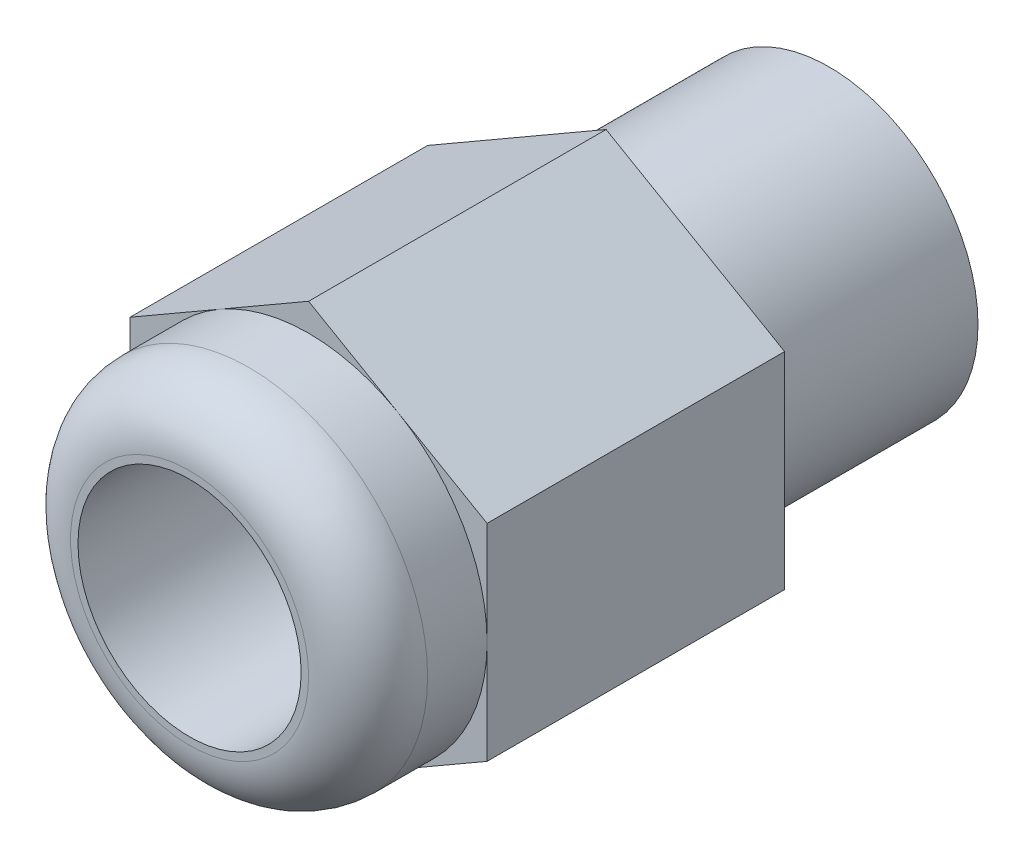
from build123d import *
from build123d.topology import SkipClean

# Parameters (mm, degrees)
SKETCH_1_R      = 7.5
EXTRUDE_1_DEPTH = 20
SKETCH_3_R      = 12
SKETCH_3_R_2    = 7.5
EXTRUDE_3_DEPTH = 8
FILLET_1_R      = 4
EXTRUDE_START   = 15
SKETCH_4_R      = 10
SKETCH_4_R_2    = 7.5
EXTRUDE_4_DEPTH = 15


with BuildPart() as part:
    # 草图1 → 凸台-拉伸1 (new body)
    with BuildSketch(Plane.XY):
        Polygon((0, 13.856406461), (-12, 6.92820323), (-12, -6.92820323), (0, -13.856406461), (12, -6.92820323), (12, 6.92820323), align=None)
        Circle(SKETCH_1_R, mode=Mode.SUBTRACT)
    extrude(amount=EXTRUDE_1_DEPTH)

    # 草图3 → 凸台-拉伸3 (add)
    with BuildSketch(Plane.XY.offset(20)):
        Circle(SKETCH_3_R)
        Circle(SKETCH_3_R_2, mode=Mode.SUBTRACT)
    extrude(amount=EXTRUDE_3_DEPTH)

    # 圆角1
    fillet_1_edges = [part.edges().sort_by_distance(p)[0] for p in [
        (-12, 0, 28),
    ]]
    fillet(fillet_1_edges, radius=FILLET_1_R)

    # 草图4 → 凸台-拉伸4 (add)
    with SkipClean():  # the faces are left unmerged after this step: merging them gives an invalid solid
        with BuildSketch(Plane(origin=(0, 0, 0), x_dir=(-1, 0, 0), z_dir=(0, 0, -1)).offset(EXTRUDE_START)):
            with Locations(Location((0, 0, 0), (0, 0, 180))):
                Circle(SKETCH_4_R)
            Circle(SKETCH_4_R_2, mode=Mode.SUBTRACT)
        extrude(amount=-EXTRUDE_4_DEPTH)


solid = part.part
